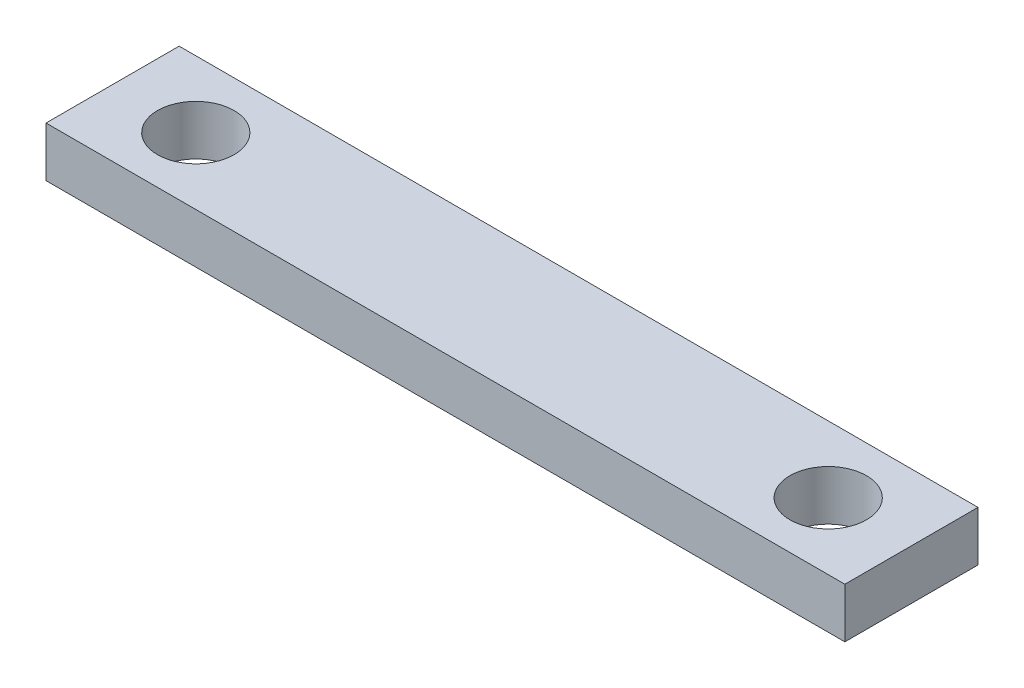
SolidWorks part; units mm, degrees
ref_plane "Front Plane" through (0, 0, 0) normal (0, 0, 1) x (1, 0, 0)
ref_plane "Top Plane" through (0, 0, 0) normal (0, 1, 0) x (1, 0, 0)
ref_plane "Right Plane" through (0, 0, 0) normal (1, 0, 0) x (0, 0, -1)
sketch "Sketch1" plane through (0, 0, 0) normal (0, 1, 0) x (1, 0, 0)
  line L1 (-12, 2) -> (12, 2)
  line L2 (-12, 2) -> (-12, -2)
  line L3 (-12, -2) -> (12, -2)
  line L4 (12, 2) -> (12, -2)
  line L5 (-12, 2) -> (12, -2) construction
  line L6 (-12, -2) -> (12, 2) construction
  point P0 (0, 0)
  dimension "D1" = 24
  dimension "D2" = 4
extrude "Boss-Extrude1" add sketch "Sketch1" along normal mid plane 1.5
hole_wizard "Ø2.3 (2.3) Diameter Hole1" positions "Sketch3" profile "Sketch2" hole size "Ø2.3" standard "Gb" end condition through all
sketch "Sketch3" plane through (0, 0.75, 0) normal (0, 1, 0) x (1, 0, 0)
  line L0 (0, 0) -> (0, 3.4746) construction
  line L2 (-12, 2) -> (-12, -2) construction
  point P0 (-9.5, 0)
  point P2 (9.5, 0)
  dimension "D1" = 2.5
sketch "Sketch2" plane through (-9.5, 0.75, 0) normal (1, 0, 0) x (0, 0, 1)
  line L0 (0, 0) -> (0, 1.5)
  line L1 (0, 1.5) -> (1.15, 1.5)
  line L2 (1.15, 1.5) -> (1.15, 0)
  line L5 (1.15, 0) -> (0, 0)
  line L11 (0, -6.35) -> (0, 107.95) construction
  dimension "通孔孔直径" = 2.3
  dimension "通孔孔深度" = 1.5
